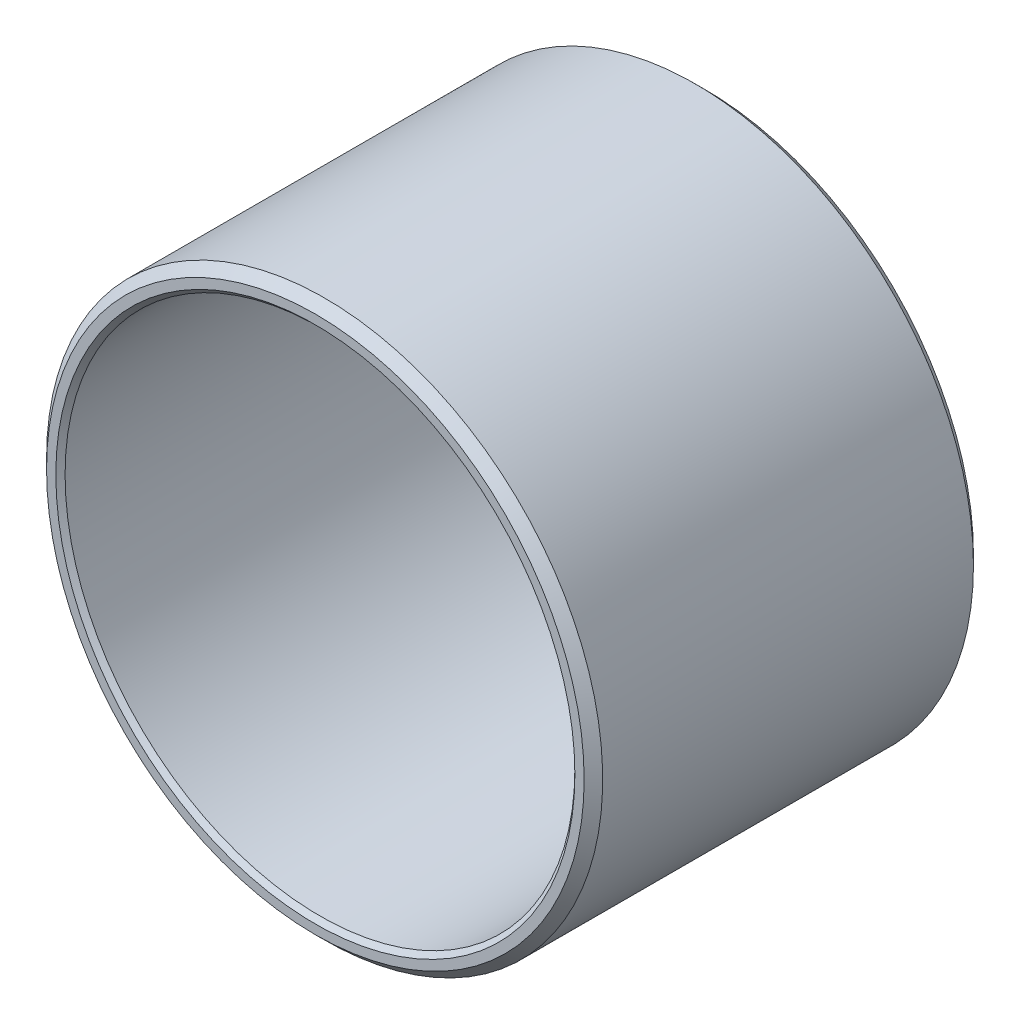
SolidWorks part; units mm, degrees
material "20钢"
ref_plane "Front Plane" through (0, 0, 0) normal (0, 0, 1) x (1, 0, 0)
ref_plane "Top Plane" through (0, 0, 0) normal (0, 1, 0) x (1, 0, 0)
ref_plane "Right Plane" through (0, 0, 0) normal (1, 0, 0) x (0, 0, -1)
sketch "Sketch1" plane through (0, 0, 0) normal (0, 0, 1) x (1, 0, 0)
  circle A0 centre (0, 0) radius 55
  circle A1 centre (0, 0) radius 60
  dimension "D1" = 110
  dimension "D2" = 120
extrude "Boss-Extrude1" add sketch "Sketch1" along normal mid plane 84
chamfer "Chamfer1" distance 2 angle 45 2 edges at (60, 0, 42) (60, 0, -42)
chamfer "Chamfer2" distance 1 angle 45 2 edges at (55, 0, -42) (55, 0, 42)
